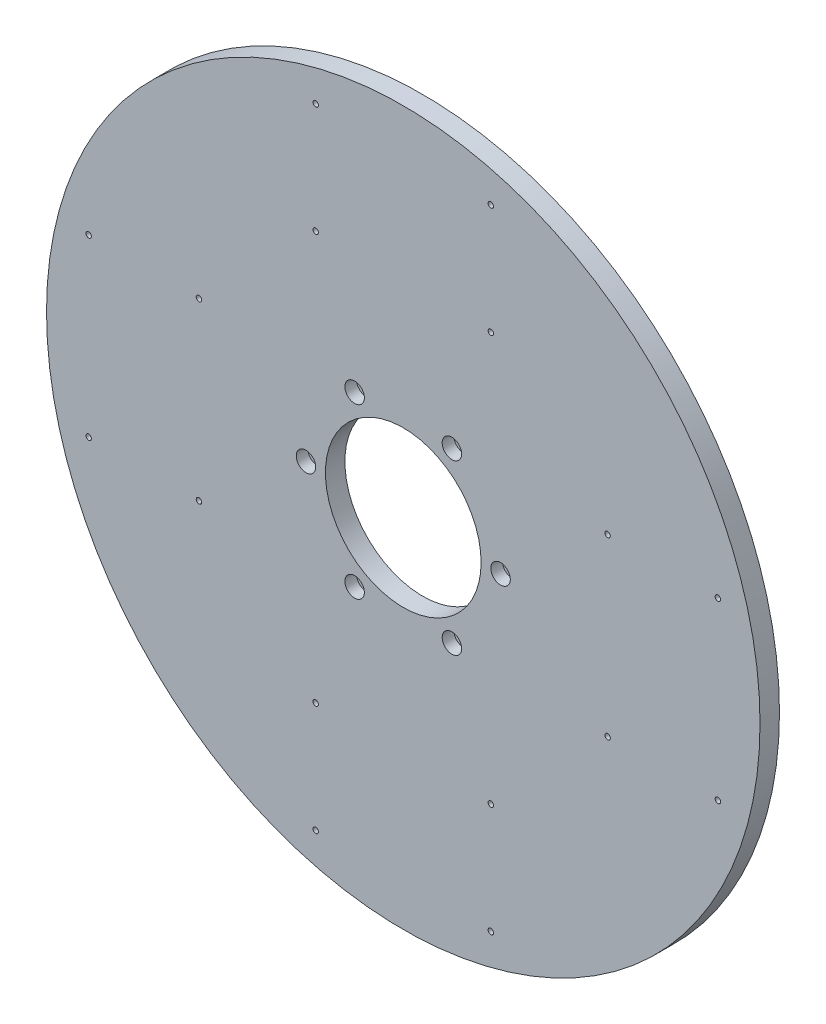
from build123d import *

# Parameters (mm, degrees)
SKETCH1_R                                         = 275
BOSS_EXTRUDE1_DEPTH                               = 15
SKETCH2_R                                         = 60
CUT_EXTRUDE1_DEPTH                                = 390.197893108
M5_TAPPED_HOLE1_D                                 = 4.2
CIRPATTERN1_COUNT                                 = 4
HOLE_SIZE_BASED_SOCKET_HEAD_CAP_SCREW_D           = 9
HOLE_SIZE_BASED_SOCKET_HEAD_CAP_SCREW_CBORE_D     = 15
HOLE_SIZE_BASED_SOCKET_HEAD_CAP_SCREW_CBORE_DEPTH = 9
CIRPATTERN2_COUNT                                 = 6


with BuildPart() as part:
    # Sketch1 → Boss-Extrude1 (new body)
    with BuildSketch(Plane.XY):
        Circle(SKETCH1_R)
    extrude(amount=BOSS_EXTRUDE1_DEPTH)

    # Sketch2 → Cut-Extrude1 (cut, through all)
    with BuildSketch(Plane.XY.offset(15)):
        Circle(SKETCH2_R)
    extrude(amount=-CUT_EXTRUDE1_DEPTH, mode=Mode.SUBTRACT)

    # M5 Tapped Hole1 (through all)
    with Locations(Plane.XY.offset(15)):
        with Locations((67.5, 157.5), (67.5, 242.5), (-67.5, 157.5), (-67.5, 242.5)):
            m5_tapped_hole1 = Hole(M5_TAPPED_HOLE1_D / 2)

    # CirPattern1: M5 Tapped Hole1 ×4 about axis
    cirpattern1_axis = Axis((0, 0, 0), (0, 0, 1))
    for i in range(1, CIRPATTERN1_COUNT):
        add(m5_tapped_hole1.rotate(cirpattern1_axis, i * 360 / CIRPATTERN1_COUNT), mode=Mode.SUBTRACT)

    # Hole Size (%based) Socket Head Cap Screw Type1 (through all)
    with Locations(Plane.XY.offset(15)):
        with Locations((-37.5, 64.951905284)):
            hole_size_based_socket_head_cap_screw = CounterBoreHole(HOLE_SIZE_BASED_SOCKET_HEAD_CAP_SCREW_D / 2, HOLE_SIZE_BASED_SOCKET_HEAD_CAP_SCREW_CBORE_D / 2, HOLE_SIZE_BASED_SOCKET_HEAD_CAP_SCREW_CBORE_DEPTH)

    # CirPattern2: Hole Size (%based) Socket Head Cap Screw Type1 ×6 about axis
    cirpattern2_axis = Axis((0, 0, 0), (0, 0, 1))
    for i in range(1, CIRPATTERN2_COUNT):
        add(hole_size_based_socket_head_cap_screw.rotate(cirpattern2_axis, i * 360 / CIRPATTERN2_COUNT), mode=Mode.SUBTRACT)


solid = part.part
